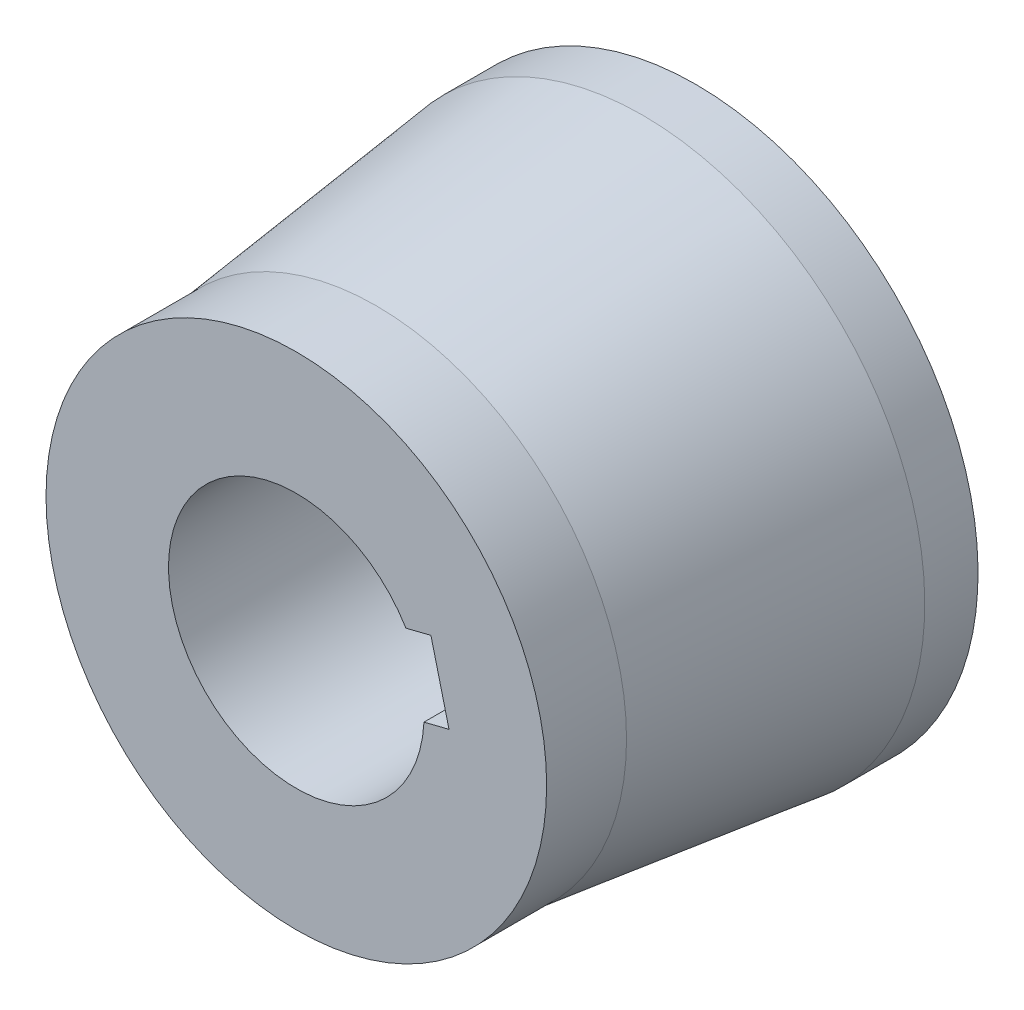
from build123d import *

# Parameters (mm, degrees)
CUT_EXTRUDE1_DEPTH = 647.654791602
SKETCH3_W          = 24
SKETCH3_H          = 75


with BuildPart() as part:
    # Sketch1 → Revolve1 (revolve)
    with BuildSketch(Plane.XZ.offset(-234.743963655), mode=Mode.PRIVATE) as revolve1_sk:
        Polygon((568.230642584, -1074.998443067), (521.230642584, -1074.998443067), (521.230642584, -1149.998443067), (574.230642584, -1149.998443067), (574.230642584, -1139.998443067), (568.230642584, -1089.998443067), align=None)
    revolve(revolve1_sk.sketch.rotate(Axis((521.230642584, 234.743963655, -1074.998443067), (0, 0, -1)), 270), axis=Axis((521.230642584, 234.743963655, -1074.998443067), (0, 0, -1)))

    # Sketch2 → Cut-Extrude1 (cut, through all)
    with BuildSketch(Plane.XY.offset(-1074.998443067)):
        with BuildLine():
            Line((549.898349026, 234.692901362), (546.50406086, 248.275198952))
            Line((546.50406086, 248.275198952), (541.805052122, 247.10089176))
            ThreePointArc((541.805052122, 247.10089176), (544.514581311, 240.562743369), (545.199340288, 233.518594169))
            Line((545.199340288, 233.518594169), (549.898349026, 234.692901362))
        make_face()
    extrude(amount=-CUT_EXTRUDE1_DEPTH, mode=Mode.SUBTRACT)

    # Sketch3 → Cut-Revolve1 (revolve, cut)
    with BuildSketch(Plane.XZ.offset(-234.743963655)):
        with Locations((533.230642584, -1112.498443067)):
            Rectangle(SKETCH3_W, SKETCH3_H)
    revolve(axis=Axis((521.230642584, 234.743963655, -1074.998443067), (0, 0, -1)), mode=Mode.SUBTRACT)


solid = part.part
